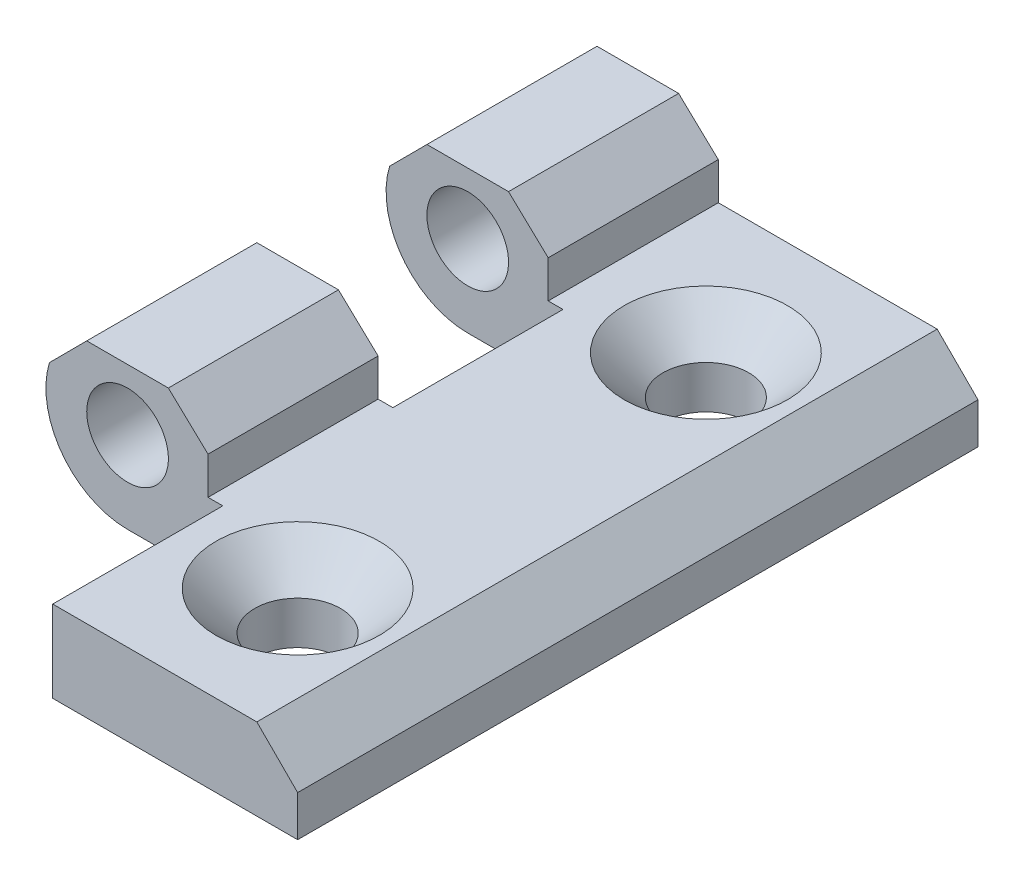
from build123d import *

# Parameters (mm, degrees)
SKETCH_1_R                = 3
EXTRUDE_1_DEPTH           = 25
CHAMFER_1_SIZE            = 3
SKETCH_2_R                = 1.072137289
CUT_EXTRUDE_1_DEPTH       = 50
HOLE_WIZARD_1_D           = 6.3
HOLE_WIZARD_1_CSINK_D     = 12
HOLE_WIZARD_1_CSINK_ANGLE = 90
SKETCH_4_W                = 23.881095176
SKETCH_4_H                = 12.5
SKETCH_4_W_2              = 26.910691004
CUT_EXTRUDE_2_DEPTH       = 50


with BuildPart() as part:
    # 草图1 → 拉伸1 (new, symmetric)
    with BuildSketch(Plane.XY):
        with BuildLine():
            Line((-7, 1), (0, 1))
            Line((0, 1), (0, 0))
            Line((0, 0), (18, 0))
            Line((18, 0), (18, 6))
            Line((18, 6), (-1.083920217, 6))
            Line((-1.083920217, 6), (-1.083920217, 8.748346358))
            Line((-1.083920217, 8.748346358), (-4, 11.5))
            Line((-4, 11.5), (-10, 11.5))
            Line((-10, 11.5), (-12.739624118, 8.748346358))
            ThreePointArc((-12.739624118, 8.748346358), (-11.821310929, 3.428591185), (-7, 1))
        make_face()
        with Locations((-7, 7)):
            Circle(SKETCH_1_R, mode=Mode.SUBTRACT)
    extrude(amount=EXTRUDE_1_DEPTH, both=True)

    # 倒角1
    chamfer_1_edges = [part.edges().sort_by_distance(p)[0] for p in [
        (18, 6, 0),
    ]]
    chamfer(chamfer_1_edges, length=CHAMFER_1_SIZE)

    # 草图2 → 切除-拉伸1 (cut)
    with BuildSketch(Plane(origin=(0, 6, 0), x_dir=(1, 0, 0), z_dir=(0, 1, 0))):
        with Locations(Location((8, 15, 0), (0, 0, 180))):
            Circle(SKETCH_2_R)
        with Locations(Location((8, -15, 0), (0, 0, 270))):
            Circle(SKETCH_2_R)
    extrude(amount=-CUT_EXTRUDE_1_DEPTH, mode=Mode.SUBTRACT)

    # 打孔尺寸开槽半沉头螺钉的类型1 (through all)
    with Locations(Plane(origin=(8, 6, -15), x_dir=(1, 0, 0), z_dir=(0, 1, 0))):
        with Locations((0, 0), (0, -30)):
            CounterSinkHole(HOLE_WIZARD_1_D / 2, HOLE_WIZARD_1_CSINK_D / 2, counter_sink_angle=HOLE_WIZARD_1_CSINK_ANGLE)

    # 草图4 → 切除-拉伸2 (cut)
    with BuildSketch(Plane(origin=(0, 11.5, 0), x_dir=(1, 0, 0), z_dir=(0, 1, 0))):
        with Locations((-11.940547588, 6.25)):
            Rectangle(SKETCH_4_W, SKETCH_4_H)
        with Locations((-13.455345502, -18.75)):
            Rectangle(SKETCH_4_W_2, SKETCH_4_H)
    extrude(amount=-CUT_EXTRUDE_2_DEPTH, mode=Mode.SUBTRACT)


solid = part.part
